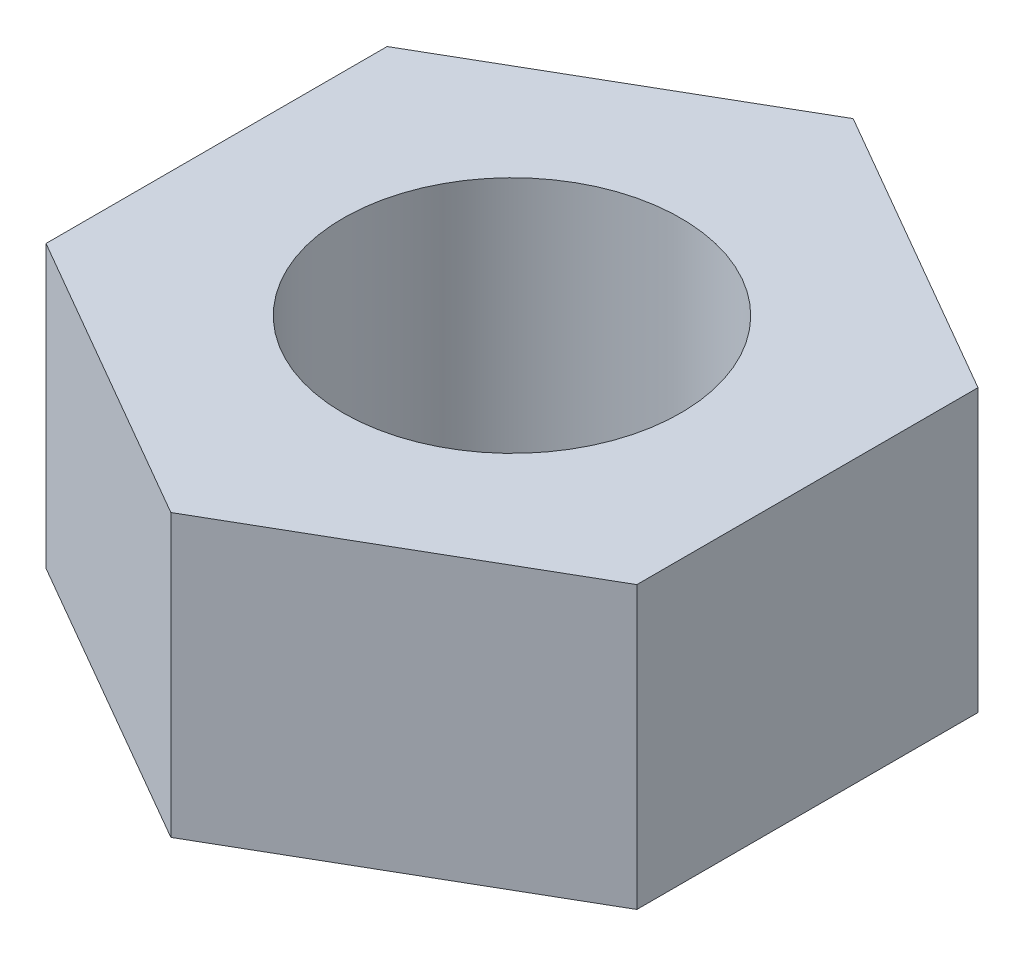
from build123d import *

# Parameters (mm, degrees)
EXTRUDE_1_DEPTH     = 10
HOLE_WIZARD_M14_1_D = 12


with BuildPart() as part:
    # 草图1 → 凸台-拉伸1 (new body)
    with BuildSketch(Plane(origin=(0, 0, 0), x_dir=(1, 0, 0), z_dir=(0, 1, 0))):
        Polygon((0, 12.124355653), (-10.5, 6.062177826), (-10.5, -6.062177826), (0, -12.124355653), (10.5, -6.062177826), (10.5, 6.062177826), align=None)
    extrude(amount=EXTRUDE_1_DEPTH)

    # M14 螺纹孔1 (through all)
    with Locations(Plane(origin=(0, 10, 0), x_dir=(1, 0, 0), z_dir=(0, 1, 0))):
        with Locations((0, 0)):
            Hole(HOLE_WIZARD_M14_1_D / 2)


solid = part.part
